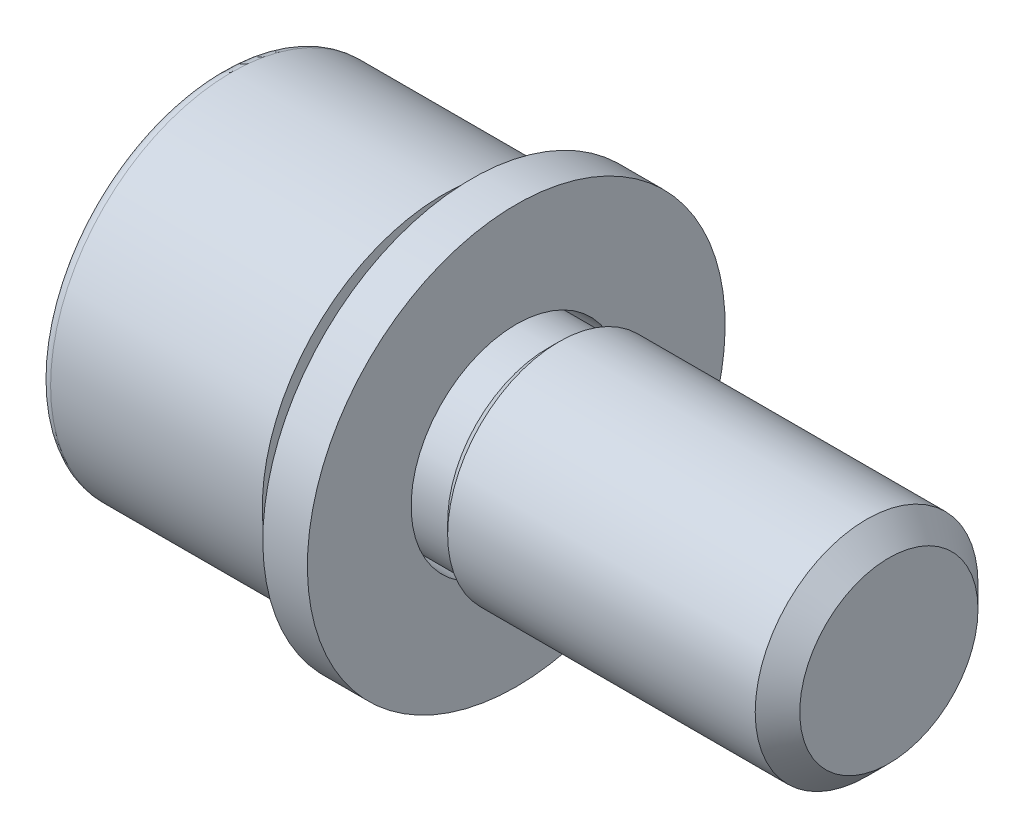
from build123d import *

# Parameters (mm, degrees)
CUT_EXTRUDE1_DEPTH = 4.7
FILLET1_R          = 0.4
SKETCH11_W         = 1.6
SKETCH11_H         = 3.725
CHAMFER1_SIZE      = 0.8


with BuildPart() as part:
    # Sketch1 → Base-Revolve (revolve)
    with BuildSketch(Plane.XY, mode=Mode.PRIVATE) as base_revolve_sk:
        with BuildLine():
            Line((0, 0), (0, 6.5))
            Line((0, 6.5), (8, 6.5))
            Line((8, 6.5), (8, 4.6))
            ThreePointArc((8, 4.6), (8.031328159, 4.444819223), (8.120405368, 4.313946086))
            Line((8.120405368, 4.313946086), (8.740405368, 3.707946086))
            ThreePointArc((8.740405368, 3.707946086), (8.869039021, 3.623580261), (9.02, 3.594))
            Line((9.02, 3.594), (11.75, 3.594))
            Line((11.75, 3.594), (12.156, 4))
            Line((12.156, 4), (24, 4))
            Line((24, 4), (24, 0))
            Line((24, 0), (0, 0))
        make_face()
    revolve(base_revolve_sk.sketch.rotate(Axis((0, 0, 0), (-1, 0, 0)), 90), axis=Axis((0, 0, 0), (-1, 0, 0)))

    # Sketch2 → Cut-Extrude1 (cut)
    with BuildSketch(Plane.ZY):
        Polygon((2.970467135, -1.715), (2.970467135, 1.715), (0, 3.43), (-2.970467135, 1.715), (-2.970467135, -1.715), (0, -3.43), align=None)
    extrude(amount=-CUT_EXTRUDE1_DEPTH, mode=Mode.SUBTRACT)

    # Sketch13 → Cut-Revolve4 (revolve, cut)
    with BuildSketch(Plane.XY):
        Polygon((0, 3.43), (0.459532865, 2.970467135), (0, 2.970467135), align=None)
    revolve(axis=Axis((0, 0, 0), (-1, 0, 0)), mode=Mode.SUBTRACT)

    # Sketch16 → Cut-Revolve5 (revolve, cut)
    with BuildSketch(Plane.XY, mode=Mode.PRIVATE) as cut_revolve5_sk:
        Polygon((6.680311423, 0), (4.7, 3.43), (4.7, 0), align=None)
    revolve(cut_revolve5_sk.sketch.rotate(Axis((4.7, 0, 0), (1, 0, 0)), 180), axis=Axis((4.7, 0, 0), (1, 0, 0)), mode=Mode.SUBTRACT)

    # Fillet1
    fillet1_edges = [part.edges().sort_by_distance(p)[0] for p in [
        (0, 0, 6.5),
    ]]
    fillet(fillet1_edges, radius=FILLET1_R)

    # Chamfer1
    chamfer1_edges = [part.edges().sort_by_distance(p)[0] for p in [
        (24, 0, 4),
    ]]
    chamfer(chamfer1_edges, length=CHAMFER1_SIZE)


with BuildPart() as body_2:
    # Sketch11 → Revolve1 (revolve)
    with BuildSketch(Plane.XY, mode=Mode.PRIVATE) as revolve1_sk:
        with Locations((9.82, 5.6375)):
            Rectangle(SKETCH11_W, SKETCH11_H)
    revolve(revolve1_sk.sketch.rotate(Axis((0, 0, 0), (1, 0, 0)), 180), axis=Axis((0, 0, 0), (1, 0, 0)))


solid = Compound([part.part, body_2.part])
